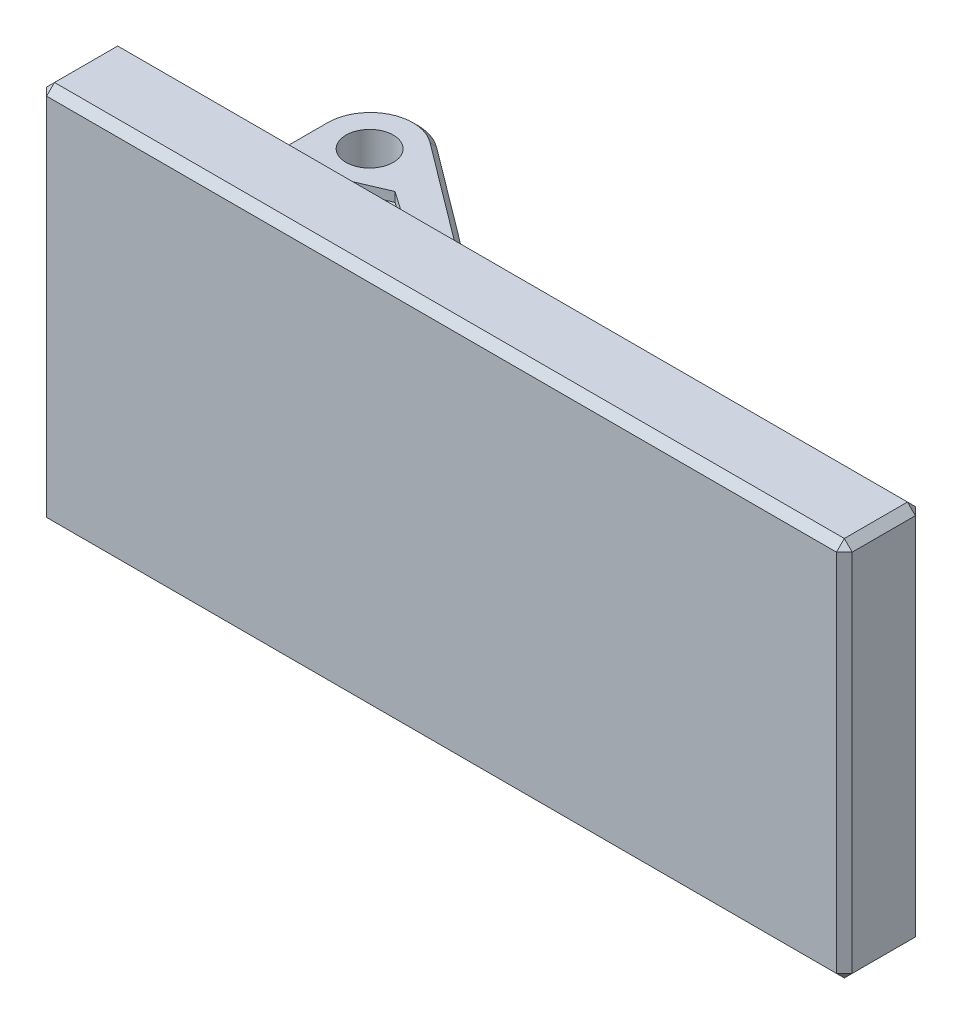
SolidWorks part; units mm, degrees
ref_plane "Front Plane" through (0, 0, 0) normal (0, 0, 1) x (1, 0, 0)
ref_plane "Top Plane" through (0, 0, 0) normal (0, 1, 0) x (1, 0, 0)
ref_plane "Right Plane" through (0, 0, 0) normal (1, 0, 0) x (0, 0, -1)
sketch "Sketch1" plane through (0, 0, 0) normal (0, 1, 0) x (1, 0, 0)
  line L0 (0, 0) -> (0, -1500)
  line L1 (0, -1500) -> (2000, -1500)
  line L2 (2000, -1500) -> (0, 0)
  circle A0 centre (306.0271, -610.083) radius 150
  dimension "D3" = 300
  dimension "D1" = 1500
  dimension "D2" = 2000
extrude "Boss-Extrude1" add sketch "Sketch1" along normal blind 1000
fillet "Fillet2" radius 300 1 edges at (0, 500, 0)
sketch "Sketch2" plane through (0, 0, 1500) normal (0, 0, 1) x (1, 0, 0)
  line L0 (0, 500) -> (6022.508, 500) construction
  line L1 (0, 1000) -> (0, 0) construction
  line L3 (-399.9514, 1705.4019) -> (4702.3059, 1705.4019)
  line L4 (-399.9514, 1705.4019) -> (-399.9514, -705.4019)
  line L5 (-399.9514, -705.4019) -> (4702.3059, -705.4019)
  line L6 (4702.3059, 1705.4019) -> (4702.3059, -705.4019)
  line L7 (-399.9514, 1705.4019) -> (4702.3059, -705.4019) construction
  line L8 (-399.9514, -705.4019) -> (4702.3059, 1705.4019) construction
  point P4 (2151.1772, 500)
extrude "Boss-Extrude2" add sketch "Sketch2" along normal blind 500
ref_plane "Plane1" through (0, 500, 0) normal (0, 1, 0) x (1, 0, 0)
ref_plane "Plane2" through (0, 800, 0) normal (0, 1, 0) x (1, 0, 0)
sketch "Sketch3" plane through (0, 800, 0) normal (0, 1, 0) x (1, 0, 0)
  line L0 (4702.3059, -1500) -> (-399.9514, -1500) construction
  line L1 (306.0271, -610.083) -> (2751.054, -1500) construction
  circle A0 centre (2751.054, -1500) radius 250
  dimension "D1" = 500
  dimension "D2" = 20
extrude "Boss-Extrude3" add sketch "Sketch3" along normal blind 200
mirror "Mirror1" about plane through (0, 500, 0) normal (0, 1, 0) of "Boss-Extrude3"
sketch "Sketch4" plane through (0, 200, 0) normal (0, 1, 0) x (1, 0, 0)
  circle A0 centre (2751.054, -1500) radius 125
  dimension "D1" = 250
extrude "Cut-Extrude1" cut sketch "Sketch4" against normal blind 150 and the other way blind 750
sketch "Sketch5" plane through (0, 0, 1500) normal (0, 0, -1) x (-1, 0, 0)
  line L0 (275, 500) -> (-275, 500) construction
  line L1 (-4590.9012, 800) -> (-3790.9012, 800)
  line L2 (-4590.9012, 800) -> (-4590.9012, 200)
  line L3 (-4590.9012, 200) -> (-3790.9012, 200)
  line L4 (-3790.9012, 800) -> (-3790.9012, 200)
  line L5 (-4590.9012, 800) -> (-3790.9012, 200) construction
  line L6 (-4590.9012, 200) -> (-3790.9012, 800) construction
  line L7 (-2501.054, 200) -> (-2626.054, 200) construction
  point P0 (-4190.9012, 500)
  dimension "D1" = 800
extrude "Cut-Extrude2" [suppressed] cut sketch "Sketch5" against normal blind 200
chamfer "Chamfer1" distance 30 angle 45 2 edges at (2751.054, 1000, 1250) (2751.054, 0, 1250)
chamfer "Chamfer2" distance 30 angle 45 6 edges at (0, 1000, 1050) (165.8359, 1000, 331.6718) (1240, 1000, 930) (0, 0, 1050) (165.8359, 0, 331.6718) (1240, 0, 930)
sketch "Sketch6" plane through (0, 1000, 0) normal (0, 1, 0) x (1, 0, 0)
  line L0 (206.7843, -1500) -> (206.7843, -941.314)
  line L1 (30, -1500) -> (1950, -1500) construction
  line L2 (206.7843, -941.314) -> (621.0429, -764.3491)
  line L3 (621.0429, -764.3491) -> (1678.8102, -1500)
  line L4 (4702.3059, -1500) -> (-399.9514, -1500) construction
  line L5 (1678.8102, -1500) -> (206.7843, -1500)
extrude "Cut-Extrude3" cut sketch "Sketch6" against normal blind 60
ref_plane "Plane3" through (0, 500, 0) normal (0, 1, 0) x (1, 0, 0)
mirror "Mirror2" about plane through (0, 500, 0) normal (0, 1, 0) of "Cut-Extrude3"
chamfer "Chamfer3" distance 50 angle 45 12 edges at (4702.3059, 500, 2000) (4702.3059, 500, 1500) (2151.1772, -705.4019, 2000) (4702.3059, -705.4019, 1750) (2151.1772, -705.4019, 1500) (-399.9514, 500, 2000) (-399.9514, -705.4019, 1750) (-399.9514, 500, 1500) (4702.3059, 1705.4019, 1750) (2151.1772, 1705.4019, 2000) (-399.9514, 1705.4019, 1750) (2151.1772, 1705.4019, 1500)
sketch "Sketch7" plane through (0, 0, 1500) normal (0, 0, -1) x (-1, 0, 0)
  line L0 (-2000, 970) -> (-2000, 30) construction
  line L1 (-2000, 220) -> (-718.2123, 220)
  line L2 (-2000, 220) -> (-2000, 780)
  line L3 (-2000, 780) -> (-718.2123, 780)
  line L4 (-718.2123, 220) -> (-718.2123, 780)
  line L5 (-1950, 1000) -> (-462, 1000) construction
  line L6 (-462, 0) -> (-1950, 0) construction
  dimension "D1" = 220
  dimension "D2" = 220
extrude "Cut-Extrude4" cut sketch "Sketch7" along normal through all
